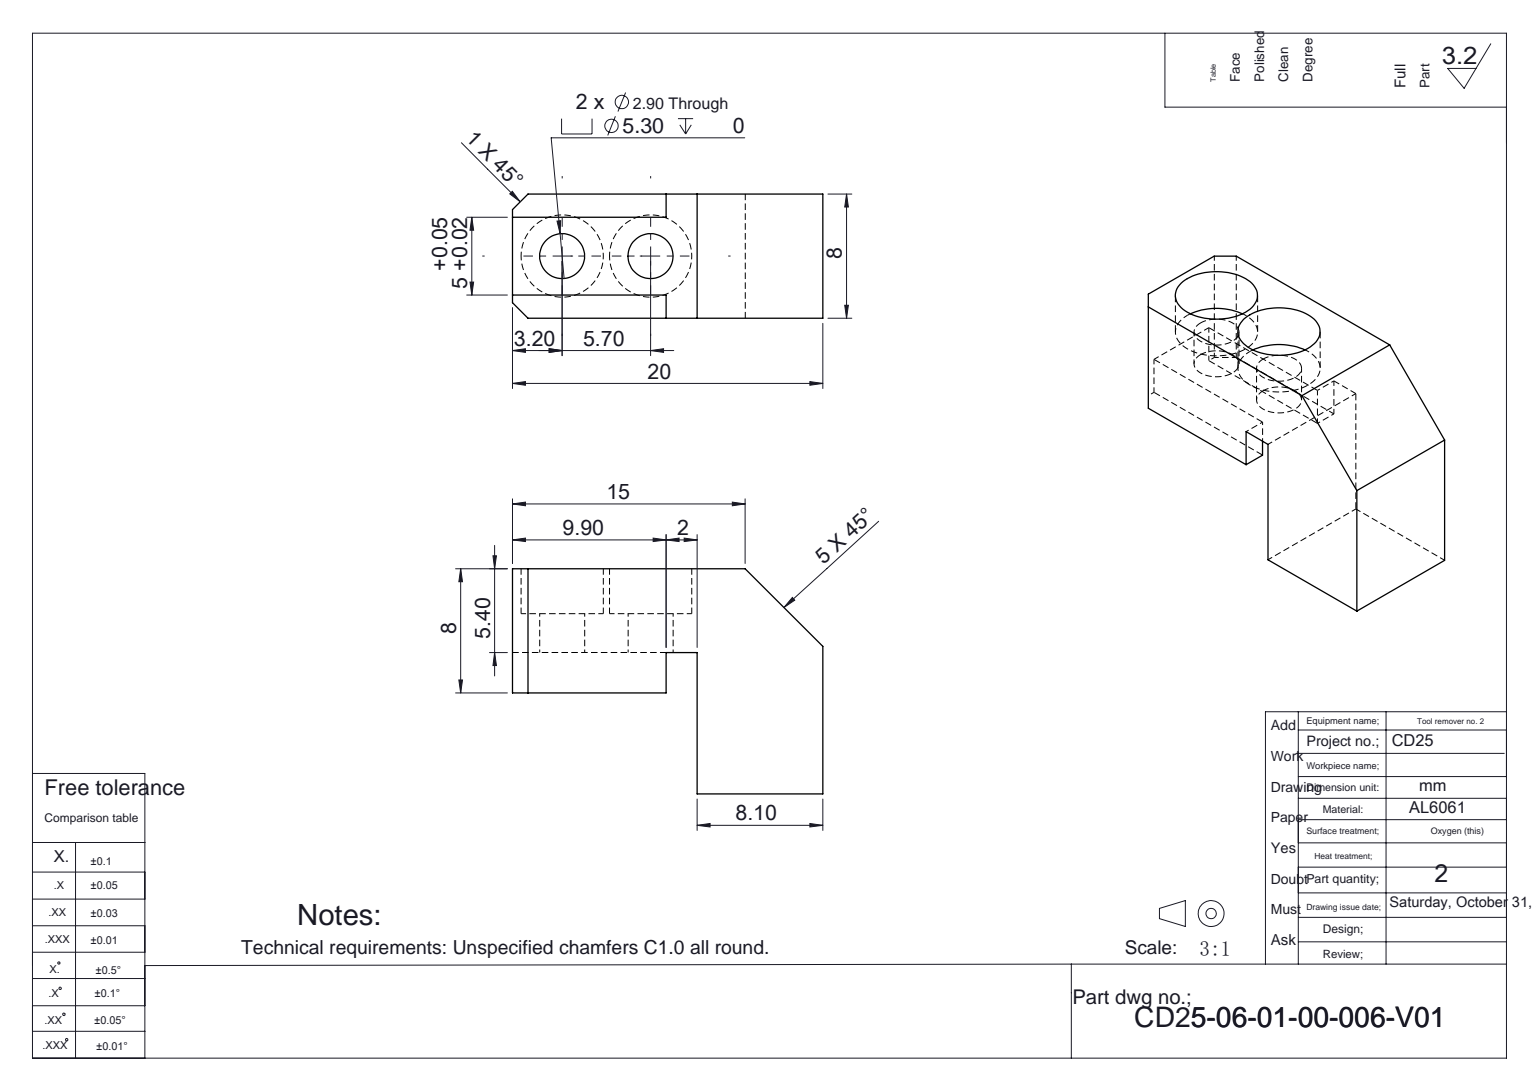
SolidWorks part; units mm, degrees
material "SUS304"
ref_plane "Front Plane" through (0, 0, 0) normal (0, 0, 1) x (1, 0, 0)
ref_plane "Top Plane" through (0, 0, 0) normal (0, 1, 0) x (1, 0, 0)
ref_plane "Right Plane" through (0, 0, 0) normal (1, 0, 0) x (0, 0, -1)
sketch "Sketch1" plane through (0, 0, 0) normal (0, 1, 0) x (1, 0, 0)
  line L1 (-4, 10) -> (4, 10)
  line L2 (-4, 10) -> (-4, -10)
  line L3 (-4, -10) -> (4, -10)
  line L4 (4, 10) -> (4, -10)
  line L5 (-4, 10) -> (4, -10) construction
  line L6 (-4, -10) -> (4, 10) construction
  point P0 (0, 0)
  dimension "D1" = 8
  dimension "D2" = 20
extrude "Boss-Extrude1" add sketch "Sketch1" along normal mid plane 14.5
sketch "Sketch2" plane through (0, -7.25, 0) normal (0, -1, 0) x (1, 0, 0)
  line L0 (-4, 10) -> (4, 10) construction
  line L1 (-2.5, 10) -> (2.5, 10)
  line L2 (-2.5, 10) -> (-2.5, -1.9)
  line L3 (-2.5, -1.9) -> (2.5, -1.9)
  line L4 (2.5, 10) -> (2.5, -1.9)
  line L5 (0, 0) -> (0, 30.5154) construction
  dimension "D1" = 5
  dimension "D2" = 11.9
extrude "Cut-Extrude1" cut sketch "Sketch2" against normal offset from surface (9.1 mm away) 5.4 up to face at (0, 7.25, 0)
hole_wizard "CBORE for M2.5 Hex Socket Head Cap Screw2" positions "Sketch4" profile "Sketch5" counterbore size "M2.5" standard "ISO" end condition through all
sketch "Sketch4" plane through (0, 7.25, 0) normal (0, 1, 0) x (1, 0, 0)
  line L0 (-4, -10) -> (4, -10) construction
  point P0 (0, -6.8)
  point P3 (0, -1.1)
  dimension "D1" = 5.7
  dimension "D2" = 3.2
sketch "Sketch5" plane through (0, 7.25, 6.8) normal (1, 0, 0) x (0, 0, 1)
  line L0 (0, 0) -> (0, 14.5)
  line L1 (0, 14.5) -> (1.45, 14.5)
  line L3 (1.45, 14.5) -> (1.45, 2.9)
  line L4 (1.45, 2.9) -> (2.65, 2.9)
  line L5 (2.65, 2.9) -> (2.65, 0)
  line L7 (2.65, 0) -> (0, 0)
  line L11 (0, -6.35) -> (0, 107.95) construction
  dimension "通孔孔直径" = 2.9
  dimension "通孔孔深度" = 14.5
  dimension "柱形沉头孔直径" = 5.3
  dimension "柱形沉头孔深度" = 2.9
sketch "Sketch6" plane through (0, -7.25, 0) normal (0, -1, 0) x (1, 0, 0)
  line L0 (-4, -0.9) -> (4, -0.9) construction
  line L4 (-4, 0.1) -> (4, 0.1)
  line L5 (-4, -1.9) -> (4, -1.9)
  line L6 (-2.5, -1.9) -> (2.5, -1.9) construction
  line L8 (4, 10) -> (4, -10) construction
  arc A2 (-4, 0.1) -> (-4, -1.9) centre (-4, -0.9) ccw
  arc A3 (4, -1.9) -> (4, 0.1) centre (4, -0.9) ccw
  point P2 (0, -0.9)
  dimension "D1" = 2
sketch "Sketch7" plane through (4, 0, 0) normal (1, 0, 0) x (0, 0, -1)
  line L0 (10, 7.25) -> (10, -7.25) construction
  line L1 (-10, -7.25) -> (1.4, -7.25)
  line L2 (-10, -7.25) -> (-10, -0.75)
  line L3 (-10, -0.75) -> (1.4, -0.75)
  line L4 (1.4, -7.25) -> (1.4, -0.75)
  line L5 (-10, 7.25) -> (10, 7.25) construction
  dimension "D1" = 8.6
  dimension "D2" = 8
extrude "Cut-Extrude3" cut sketch "Sketch7" against normal through all
chamfer "Chamfer1" distance 1 angle 45 2 edges at (-4, 3.25, 10) (4, 3.25, 10)
chamfer "Chamfer2" distance 5 angle 45 1 edges at (0, 7.25, -10)
extrude "Cut-Extrude4" cut sketch "Sketch6" against normal up to surface (9.1 mm away) up to face at (0, 1.85, 8.25)
